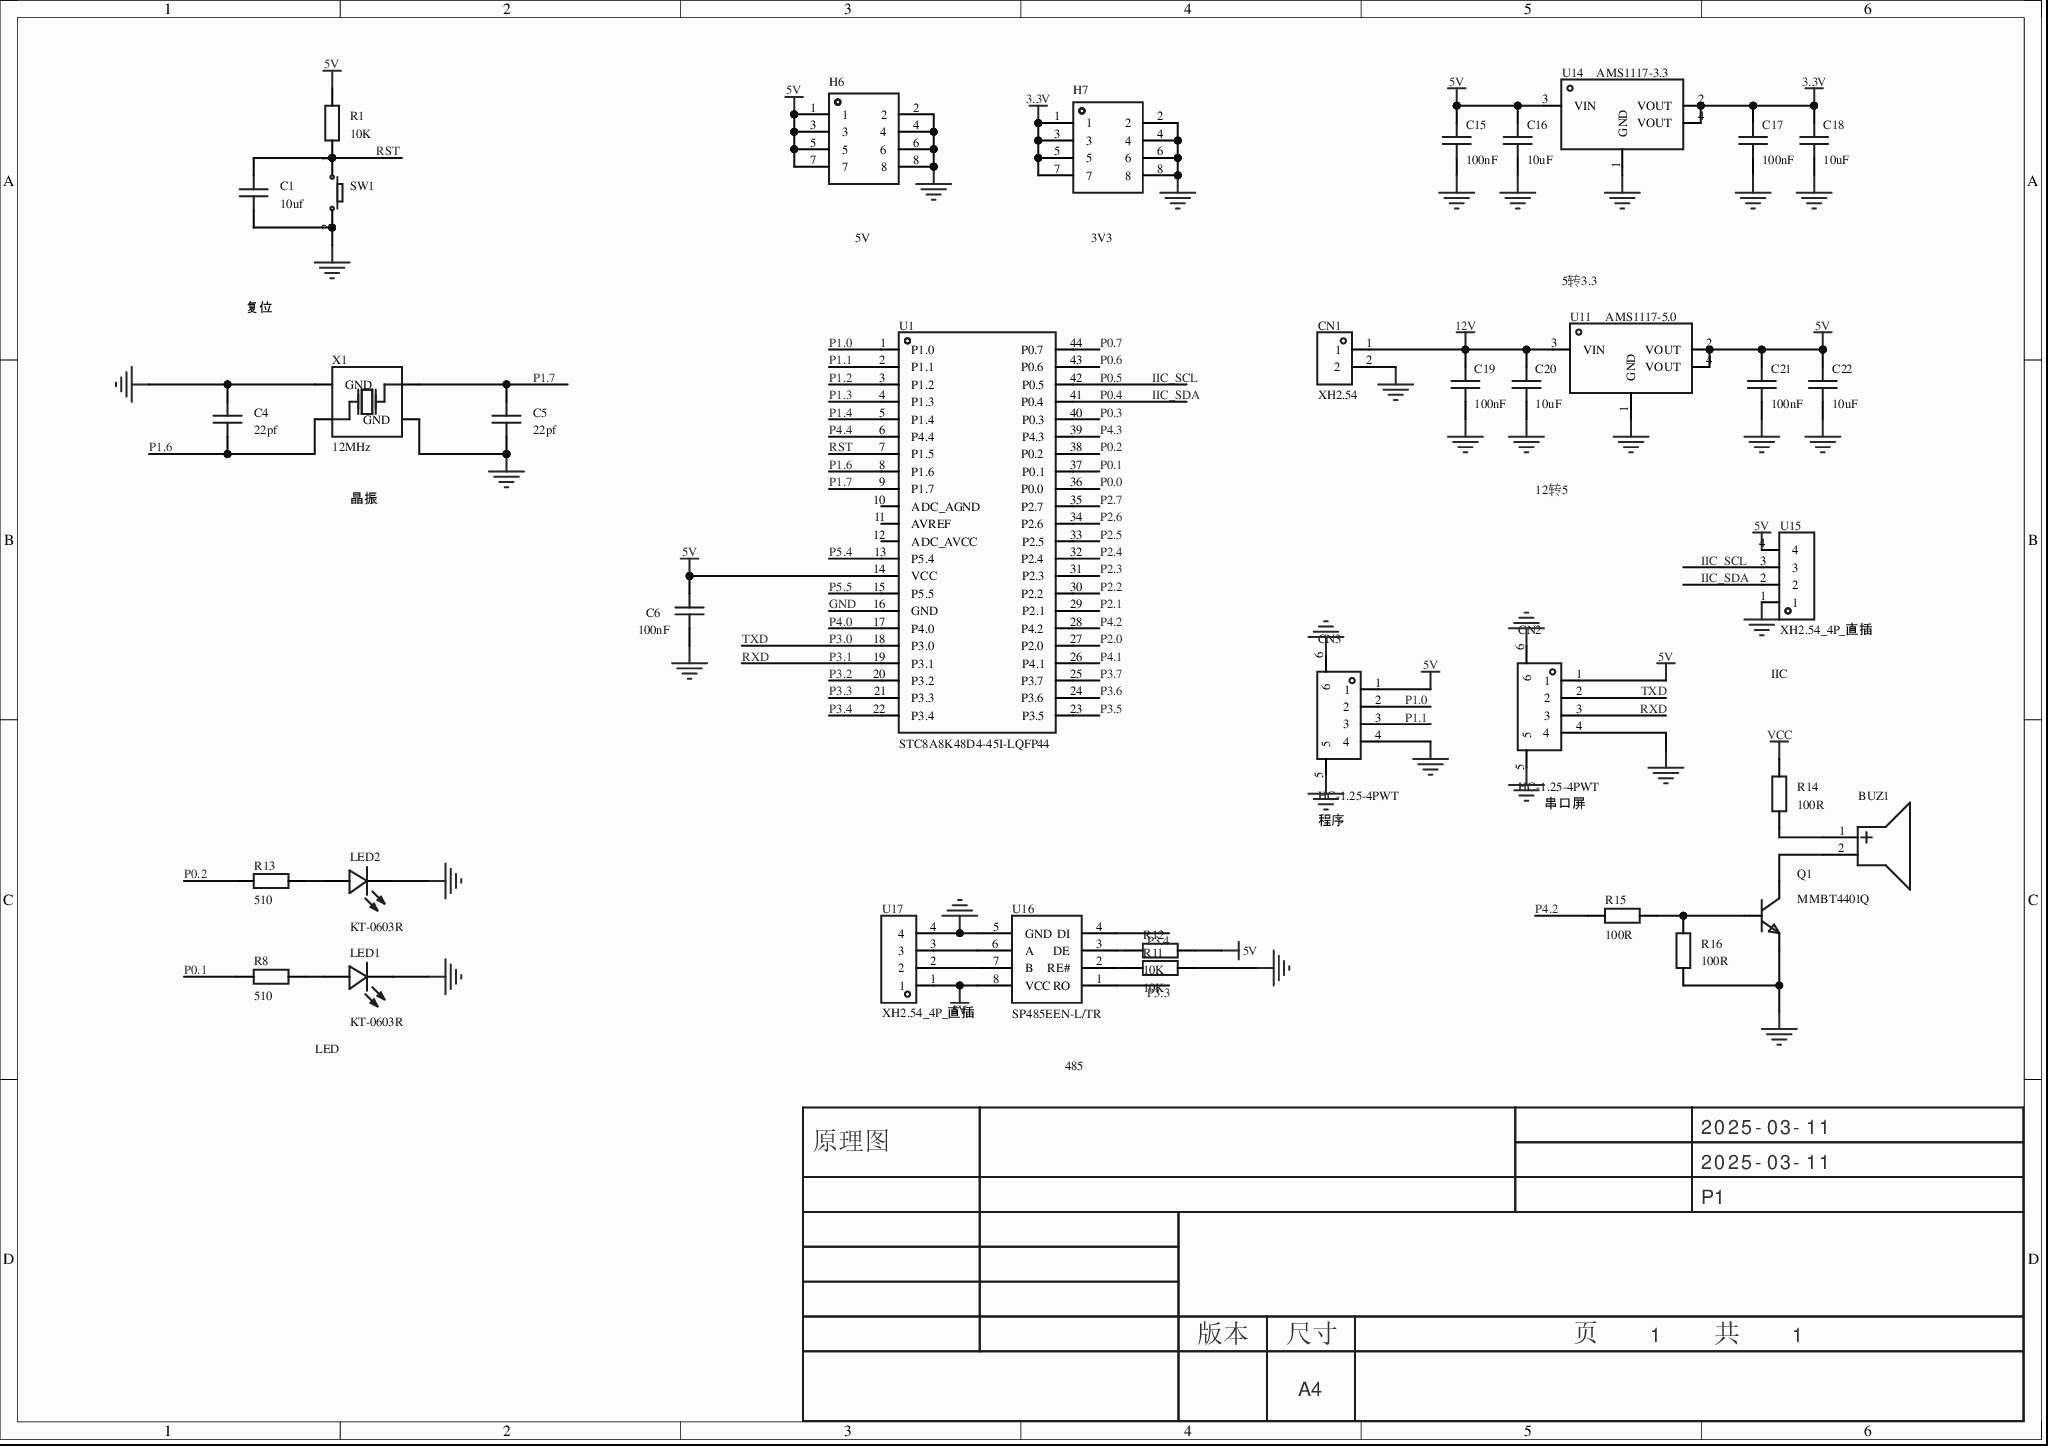
[diagram p0: MISC49860-3.schdoc]
# Altium project MISC49860-2.PrjPcb
1 sheet, 37 parts. Net scope: global (net labels, ports and power ports of the same name join across sheets).
Board file: MISC49860.pcbdoc

## Sheet MISC49860-3.schdoc
size 297 x 209 mm; Version: V1.0; @Project Name: MISC49860; @Page Count: 1; @Update Date: 2025-03-11; @Create Date: 2025-03-11; @Schematic Name: MISC49860; @Page No: 1; @Create Time: 19:24:41; @Update Time: 19:59:04; @Board Name: MISC49860

### Parts
BUZ1  5VDC蜂鸣器,Φ12,脚距7.6  [BUZ-TH_BD12.0-P7.60-D0.6-FD]  (value not drawn)
C1  10uf  [C0805]
C4  22pf  [C0805]
C5  22pf  [C0805]
C6  100nF  [C0805]
C15  100nF  [C0603]
C16  10uF  [C0603]
C17  100nF  [C0603]
C18  10uF  [C0603]
C19  100nF  [C0603]
C20  10uF  [C0603]
C21  100nF  [C0603]
C22  10uF  [C0603]
CN1  XH2.54  [CONN-TH_XH2.54-2P]
CN2  HC-1.25-4PWT  [CONN-SMD_4P-P1.25-HC-1.25-4PWT]
CN3  HC-1.25-4PWT  [CONN-SMD_4P-P1.25-HC-1.25-4PWT]
H6  (no value)  [HDR-TH_8P-P2.54-V-M-R2-C4-S2.54]
H7  (no value)  [HDR-TH_8P-P2.54-V-M-R2-C4-S2.54]
LED1  KT-0603R  [LED0603-RD]
LED2  KT-0603R  [LED0603-RD]
Q1  MMBT4401Q  [SOT-23-3_L2.9-W1.3-P1.90-LS2.4-BR]
R1  10K  [R0805]
R8  510  [R0603]
R11  10K  [R0805]
R12  10K  [R0805]
R13  510  [R0603]
R14  100R  [R0805]
R15  100R  [R0805]
R16  100R  [R0805]
SW1  (no value)  [Key_SMD_3x4x2]
U1  STC8A8K48D4-45I-LQFP44  [LQFP-44_L10.0-W10.0-P0.80-LS12.0-BL]
U11  AMS1117-5.0  [SOT-223_L6.5-W3.5-P2.30-LS7.0-BR]
U14  AMS1117-3.3  [SOT-223-3_L6.5-W3.4-P2.30-LS7.0-BR]
U15  XH2.54_4P_直插  [CONN-TH_4P-P2.50-XH2.54-4P]
U16  SP485EEN-L/TR  [SOIC-8_L5.0-W4.0-P1.27-LS6.0-BL]
U17  XH2.54_4P_直插  [CONN-TH_4P-P2.50-XH2.54-4P]
X1  12MHz  [OSC-SMD_4P-L3.2-W2.5-BL]

### Nets
3.3V: C17.2 C18.2 H7.1 H7.3 H7.5 H7.7 U14.2(VOUT) U14.4(VOUT)
5V: C6.2 C15.2 C16.2 C21.2 C22.2 CN2.1 CN3.1 H6.1 H6.3 H6.5 H6.7 R1.1 R12.2 U1.14(VCC) U11.2(VOUT) U11.4(VOUT) U14.3(VIN) U15.4 U16.8(VCC) U17.1
12V: C19.2 C20.2 CN1.1 U11.3(VIN)
GND: C1.2 C4.2 C5.1 C6.1 C15.1 C16.1 C17.1 C18.1 C19.1 C20.1 C21.1 C22.1 CN1.2 CN2.4 CN2.5 CN2.6 CN3.4 CN3.5 CN3.6 H6.2 H6.4 H6.6 H6.8 H7.2 H7.4 H7.6 H7.8 LED1.1(K) LED2.1(K) Q1.2(E) R11.2 R16.2 SW1.2 U1.16(GND) U11.1(GND) U14.1(GND) U15.1 U16.5(GND) U17.4 X1.2(GND) X1.4(GND)
VCC: R14.1
IIC_SCL: U1.42(P0.5) U15.3  [also labelled P0.5]
IIC_SDA: U1.41(P0.4) U15.2  [also labelled P0.4]
P0.0: U1.36(P0.0)
P0.1: R8.1 U1.37(P0.1)
P0.2: R13.1 U1.38(P0.2)
P0.3: U1.40(P0.3)
P0.6: U1.43(P0.6)
P0.7: U1.44(P0.7)
P1.0: CN3.2 U1.1(P1.0)
P1.1: CN3.3 U1.2(P1.1)
P1.2: U1.3(P1.2)
P1.3: U1.4(P1.3)
P1.4: U1.5(P1.4)
P1.6: C4.1 U1.8(P1.6) X1.1(OSC1)
P1.7: C5.2 U1.9(P1.7) X1.3(OSC2)
P2.0: U1.27(P2.0)
P2.1: U1.29(P2.1)
P2.2: U1.30(P2.2)
P2.3: U1.31(P2.3)
P2.4: U1.32(P2.4)
P2.5: U1.33(P2.5)
P2.6: U1.34(P2.6)
P2.7: U1.35(P2.7)
P3.0: CN2.2 U1.18(P3.0)  [also labelled TXD]
P3.1: CN2.3 U1.19(P3.1)  [also labelled RXD]
P3.2: U1.20(P3.2)
P3.3: U1.21(P3.3) U16.1(RO)
P3.4: U1.22(P3.4) U16.4(DI)
P3.5: U1.23(P3.5)
P3.6: U1.24(P3.6)
P3.7: U1.25(P3.7)
P4.0: U1.17(P4.0)
P4.1: U1.26(P4.1)
P4.2: R15.1 U1.28(P4.2)
P4.3: U1.39(P4.3)
P4.4: U1.6(P4.4)
P5.4: U1.13(P5.4)
P5.5: U1.15(P5.5)
RST: C1.1 R1.2 SW1.1 U1.7(P1.5)
NetBUZ1_1: BUZ1.1(+) R14.2
NetBUZ1_2: BUZ1.2(-) Q1.3(C)
NetLED1_2: LED1.2(A) R8.2
NetLED2_2: LED2.2(A) R13.2
NetQ1_1: Q1.1(B) R15.2 R16.1
NetR11_1: R11.1 U16.2(RE#)
NetR12_1: R12.1 U16.3(DE)
NetU16_6: U16.6(A) U17.3
NetU16_7: U16.7(B) U17.2

Not connected (* = marked no-connect by the designer): U1 10(ADC_AGND) 11(AVREF) 12(ADC_AVCC)

### Notes on the sheet
- (near H6) 5V
- (near H7) 3V3
- 复位
- 5转3.3
- 晶振
- 12转5
- IIC
- (near CN3) 程序
- (near CN2) 串口屏
- LED
- 485
- 2025-03-11
- 原理图
- P1
- 版本
- 尺寸
- A4
- 页    1    共    1

### Library data of the parts
BUZ1 = 5VDC蜂鸣器,Φ12,脚距7.6: AddInBom: yes; ModelId: 16ab50e14c5b4f2c986c135bdba60e37; ModelName: BUZ-TH_D12.0-H9.5-P7.60; ModelTransform: 472.44,472.176,0,90,0,0,-0.787,0,-177.165; Symbol: 5VDC蜂鸣器,Φ12,脚距7.6; Device: 5VDC蜂鸣器,Φ12,脚距7.6; LCSC Part Name: 5VDC蜂鸣器,Φ12,脚距7.6; SupplierPart: C9900018824; ManufacturerPart: 5VDC蜂鸣器,Φ12,脚距7.6; Supplier Footprint: BUZ-TH; JLCPCB Part Class: 扩展库; Supplier: LCSC; ConvertToPcb: yes; FootprintName: BUZ-TH_BD12.0-P7.60-D0.6-FD
C1 C4-C6 = CAP_0805: ConvertToPcb: yes; SymbolName: CapAcitance; ModelId: 1ba041120af144c991958decab20d241; ModelName: C0805_L2.0-W1.3-H1.3; ModelTransform: 78.74,51.181,0,0,0,0,0,0.0005,0; Device: CAP_0805; AddInBom: yes; Supplier Footprint: 0805; FootprintName: C0805
  C1: Value: 10uf
  C4 C5: Value: 22pf
  C6: Value: 100nF
C15-C22 = CAP_0603: ConvertToPcb: yes; SymbolName: CapAcitance; ModelId: ac125912035d415993ca9572d50418b1; ModelName: C0603_L1.6-W0.8-H0.8; ModelTransform: 62.992,31.496,0,0,0,0,0,0,0; Device: CAP_0603; AddInBom: yes; Supplier Footprint: 0603; FootprintName: C0603
  C15 C17 C19 C21: Value: 100nF
  C16 C18 C20 C22: Value: 10uF
CN1 = XH2.54-2PIN-直针: AddInBom: yes; ModelId: dc9654a6caad4c20aab3bc231ea458cf; ModelTransform: 296.889,230.315,0,0,0,0,0,26.653,-137.795; Symbol: XH2.54-2PIN-直针; Manufacturer Part: XH2.54; Device: XH2.54-2PIN-直针; LCSC Part Name: XH2.54-2PIN-直针; SupplierPart: C9900011425; Supplier Footprint: XH2.54-2PIN; JLCPCB Part Class: 扩展库; Supplier: LCSC; ConvertToPcb: yes; FootprintName: CONN-TH_XH2.54-2P; ModelName: CONN-TH_XH2.54-2P
CN2 CN3 = HC-1.25-4PWT: 插针结构:1x4P;间距:1.25mm;安装方式:卧贴;参考系列:PicoBlade(MX 1.25);总PIN数:4P;排数:1;每排PIN数:4;行距:-;额定电流:1A;触头材质:黄铜;触头镀层:锡;工作温度范围:-40℃~+105℃;; Manufacturer: HCTL(华灿天禄); AddInBom: yes; ModelId: a5d89d01fe1c41f780224f4e5aebbf3c; ModelTransform: 393.7,206.693,0,0,0,0,-0.001,-39.372,0; Pins Structure: 1x4P; Pitch: 1.25mm; Number of PINs Per Row: 4; Current Rating (Max): 1A; Rated Voltage (Max): 125V; Plastic Material: LCP; Flame Retardant Rating: UL94V-0; Supplementary Features: 辅助焊脚; Z-Height of the Board: 3.57mm; X-Length of Bottom Edge on Board (Spacing Line): 10.05mm; Y-Width of Bottom Edge on Board: 5.25mm; Symbol: HC-1.25-4PWT; Device: HC-1.25-4PWT; LCSC Part Name: 1x4P 间距:1.25mm 卧贴 系列:PicoBlade(MX 1.25); SupplierPart: C2845381; ManufacturerPart: HC-1.25-4PWT; Supplier Footprint: SMD,P=1.25mm,卧贴; JLCPCB Part Class: 扩展库; Datasheet: https://atta.szlcsc.com/upload/public/pdf/source/20240930/9508A8292CCC87B0C29E3A028D56E30A.pdf; Supplier: LCSC; ConvertToPcb: yes; FootprintName: CONN-SMD_4P-P1.25-HC-1.25-4PWT; ModelName: CONN-SMD_4P-P1.25-HC-1.25-4PWT; Mounting Style: 卧贴; Reference Series: PicoBlade(MX 1.25); Number of Pins: 4P; Number of Rows: 1; Row Spacing: -; Contact Material: 黄铜; Contact Plating: 锡; Operating Temperature Range: -40℃~+105℃; Colour: -
H6 H7 = HDR-M_2.54_2x4: Symbol: HDR-M-2.54_2x4; ConvertToPcb: yes; ModelId: 9655140a9899454ea9d6a6732d55fb0e; ModelName: HDR-TH_8P-P2.54-M-LI-2X4P; ModelTransform: 399.999,200,0,0,0,0,0,0,-118.11; Device: HDR-M_2.54_2x4; AddInBom: yes; SupplierPart: C124386; Supplier Footprint: 插件,P=2.54mm; FootprintName: HDR-TH_8P-P2.54-V-M-R2-C4-S2.54
LED1 LED2 = KT-0603R: 发光颜色:红色;功率:-;正向电流:-;主波长:-;二极管配置:-;透镜颜色:-;色温:-;发光角度:-;载带方式:-;工作温度:-40℃~+85℃;; Manufacturer: KENTO; AddInBom: yes; ModelId: 1f0d29a91be547639d425604e9b96ebb; ModelTransform: 63.7794,32.283,0,0,0,0,0,0,0; Emitted Color: 红色; Symbol: KT-0603R; Device: KT-0603R; LCSC Part Name: 0603 红灯 高亮; SupplierPart: C2286; ManufacturerPart: KT-0603R; Supplier Footprint: 0603; JLCPCB Part Class: 基础库; Datasheet: https://atta.szlcsc.com/upload/public/pdf/source/20160616/1466072038404.pdf; Supplier: LCSC; ConvertToPcb: yes; FootprintName: LED0603-RD; ModelName: LED0603-RD; Power Dissipation: -; Forward Current: -; Dominant Wavelength: -; Peak Wavelength: -; Diode Configuration: -; Lens Color: -; Color Temperature: -; Viewing Angle: -; Mounting Sytle: -; Operating Temperature: -40℃~+85℃
Q1 = MMBT4401Q: 晶体管类型:NPN;集电极电流(Ic):600mA;集射极击穿电压(Vceo):40V;耗散功率(Pd):300mW;直流电流增益(hFE):100@150mA,1V;; Manufacturer: YANGJIE(扬杰); AddInBom: yes; ModelId: c62791f0466c4ae2a892c056b845b0ca; ModelName: SOT-23-3P_L2.9-W1.3-H1.0-LS2.4-P0.95; ModelTransform: 98.425,114.173,0,180,0,0,0.0005,-0.0005,0; type: NPN; Current - Collector(Ic): 600mA; Collector - Emitter Voltage VCEO: 40V; Pd - Power Dissipation: 300mW; Transition frequency(fT): 250MHz; Current - Collector Cutoff: 100nA; Vce Saturation(VCE(sat)): 400mV@150mA,15mA; Symbol: MMBT4401Q; Device: MMBT4401Q; LCSC Part Name: MMBT4401Q; SupplierPart: C699219; ManufacturerPart: MMBT4401Q; Supplier Footprint: SOT-23(TO-236); JLCPCB Part Class: 扩展库; Datasheet: https://atta.szlcsc.com/upload/public/pdf/source/20200709/C699219_5916070C8AE9E936AEED1A6139F8D2E4.pdf; Supplier: LCSC; ConvertToPcb: yes; FootprintName: SOT-23-3_L2.9-W1.3-P1.90-LS2.4-BR; DC Current Gain: 100@150mA,1V; Operating Temperature: -55℃~+150℃
R1 R11 R12 R14-R16 = Res_0805: Symbol: 电阻; ConvertToPcb: yes; ModelId: 37a81e68749a4138bd2dfa6897b24b85; ModelName: R0805_L2.0-W1.3-H0.6; ModelTransform: 78.74,51.181,0,0,0,0,0,-0.0005,0; Device: Res_0805; AddInBom: yes; Supplier Footprint: 0805; FootprintName: R0805
  R1 R11 R12: Value: 10K
  R14-R16: Value: 100R
R8 R13 = Res_0603: ConvertToPcb: yes; SymbolName: 电阻; ModelId: fc143cca1e79419f9cd78b61e9279f08; ModelTransform: 31.8897,63.7794,0,90,0,0,0,0,0; Value: 510; Device: Res_0603; AddInBom: yes; Supplier Footprint: 0603; FootprintName: R0603; ModelName: R0603
SW1 = Key_SMD_3x4x2: ConvertToPcb: yes; SymbolName: 轻触按键x2; ModelId: 63599cce708d48afbce1b0db003544770819f05c4eef4c71ace90d822a990e87; ModelName: SW-SMD_L4.0-W2.9-H2-LS5.0; ModelTransform: 196.85,114.17,79.13,0,0,0,0,0,0; Device: Key_SMD_3x4x2; AddInBom: yes; Supplier Footprint: SMD; FootprintName: Key_SMD_3x4x2
U1 = STC8A8K48D4-45I-LQFP44: Manufacturer: STC(宏晶); AddInBom: yes; ModelId: cfc67ede9fd147078f17820e55193bca; ModelName: LQFP-44_L10.0-W10.0-H1.4-LS12.0-P0.80; ModelTransform: 472.441,472.441,0,0,0,0,0,0,0; Symbol: STC8A8K48D4-45I-LQFP44; Device: STC8A8K48D4-45I-LQFP44; LCSC Part Name: STC8A8K48D4-45I-LQFP44; SupplierPart: C3013132; ManufacturerPart: STC8A8K48D4-45I-LQFP44; Supplier Footprint: LQFP-44(10x10); JLCPCB Part Class: 扩展库; Datasheet: https://atta.szlcsc.com/upload/public/pdf/source/20220509/6F36F3B8C41E8D6E23754E39225582EF.pdf; Supplier: LCSC; ConvertToPcb: yes; FootprintName: LQFP-44_L10.0-W10.0-P0.80-LS12.0-BL
U11 = AMS1117-5.0_C6187: 输出类型:固定;工作电压:12V;输出电压:5V;输出电流:1A;电源纹波抑制比(PSRR):-;输出极性:正极;; Manufacturer: AMS; AddInBom: yes; Output Type: 固定; Voltage - Supply: 12V; Output Voltage: 5V; Output Current: 1A; Voltage Dropout: 1.3V@(1A); Output Configuration: 正极; Number of Outputs: 1; ModelId: 925194bf9823436183a3e0b978a8d076; ModelName: SOT-223-4P_L6.5-W3.5-H1.6-LS7.0-P2.30; ModelTransform: 279.89794,255.905,0,180,0,0,0.0005,0.0005,0; Symbol: AMS1117-5.0; Device: AMS1117-5.0_C6187; LCSC Part Name: 输入12V 输出5V 1A; SupplierPart: C6187; ManufacturerPart: AMS1117-5.0; Supplier Footprint: SOT-223; JLCPCB Part Class: 基础库; Datasheet: https://atta.szlcsc.com/upload/public/pdf/source/20230918/E4B716057EE82179D88E8A0894830D59.pdf; Supplier: LCSC; ConvertToPcb: yes; Power Supply Rejection Ratio (PSRR): -; standby current: -; Noise: -; Features: 过流保护(OCP); Operating Temperature: -; FootprintName: SOT-223_L6.5-W3.5-P2.30-LS7.0-BR
U14 = AMS1117-3.3_C6186: 输出类型:固定;工作电压:-;输出电压:3.3V;输出电流:1A;电源纹波抑制比(PSRR):72dB@(120Hz);输出极性:正极;; Manufacturer: AMS; AddInBom: yes; Output Type: 固定; Output Voltage: 3.3V; Output Current: 1A; Voltage Dropout: 1.3V@(800mA); Output Configuration: 正极; Number of Outputs: 1; ModelId: 925194bf9823436183a3e0b978a8d076; ModelName: SOT-223-4P_L6.5-W3.5-H1.6-LS7.0-P2.30; ModelTransform: 279.89794,255.905,0,180,0,0,-3.9385,-0.0005,0; Symbol: AMS1117-3.3; Device: AMS1117-3.3_C6186; LCSC Part Name: 输出3.3V 1A; SupplierPart: C6186; ManufacturerPart: AMS1117-3.3; Supplier Footprint: SOT-223; Datasheet: https://atta.szlcsc.com/upload/public/pdf/source/20180727/C6186_7A095716F0823C02F1997A905E26C086.pdf; Supplier: LCSC; ConvertToPcb: yes; Voltage - Supply: -; Power Supply Rejection Ratio (PSRR): 72dB@(120Hz); standby current: -; Noise: -; Features: 过流保护(OCP)；热关断(TSD); Operating Temperature: -; FootprintName: SOT-223-3_L6.5-W3.4-P2.30-LS7.0-BR
U15 U17 = XH2.54_4P_直插: AddInBom: yes; ModelId: c69236e4c0a047c6aeeeefc1552045f5; ModelTransform: 492.125,228.346,0,180,0,0,0,-19.685,-137.795; Symbol: XH2.54_4P_直插; Device: XH2.54_4P_直插; LCSC Part Name: XH2.54_4P_直插; SupplierPart: C9900008616; ManufacturerPart: XH2.54_4P_直插; Supplier Footprint: XH2.54_4P; JLCPCB Part Class: 扩展库; Supplier: LCSC; ConvertToPcb: yes; FootprintName: CONN-TH_4P-P2.50-XH2.54-4P; ModelName: CONN-TH_4P-P2.50-XH2.54-4P
U16 = SP485EEN-L/TR: 类型:收发器;数据速率:10Mbps;; Manufacturer: MaxLinear(迈凌); AddInBom: yes; ModelId: e81d2f7d937b4a6ab1dca543ff5d56a4; ModelName: SOIC-8_L4.9-W3.9-H1.7-LS6.0-P1.27; ModelTransform: 189.751,236.22,0,0,0,0,-0.0005,0.0005,0; Types: 收发器; Number of Driver: 1; Supply Voltage: 4.75V~5.25V; Data Rate: 10Mbps; Symbol: SP485EEN-L/TR; Device: SP485EEN-L/TR; LCSC Part Name: 增强型低功耗半双工 RS-485 收发器; SupplierPart: C6855; ManufacturerPart: SP485EEN-L/TR; Supplier Footprint: SOIC-8; Datasheet: https://atta.szlcsc.com/upload/public/pdf/source/20210125/C916163_66C97B5ACCC910994E8B10780F9BD300.pdf; Supplier: LCSC; ConvertToPcb: yes; FootprintName: SOIC-8_L5.0-W4.0-P1.27-LS6.0-BL; Number of receiver: 1; Operating Temperature: -40℃~+85℃
X1 = 7M12000039: 晶振类型:贴片晶振;频率:12MHz;常温频差:±20ppm;外接负载电容:18pF;频率稳定度(全温):±20ppm;; Manufacturer: TXC(晶技); Symbol: 7M1209LCSC-DDJ4S; AddInBom: yes; ModelId: ae22b8d143894765bc8100c37cb6356f; ModelName: OSC-SMD_4P-L3.2-W2.5-H1.0; ModelTransform: 125.984,98.425,0,0,0,0,0,0,0; Crystal Type: 贴片晶振; Normal temperature Frequency Tolerance: ±20ppm; External load capacitor: 18pF; Equivalent Series Resistance (ESR): 100Ω; Device: 7M12000039; LCSC Part Name: 12MHz ±20ppm 18pF; SupplierPart: C90900; ManufacturerPart: 7M12000039; Supplier Footprint: SMD3225-4P; JLCPCB Part Class: 扩展库; Datasheet: https://atta.szlcsc.com/upload/public/pdf/source/20170408/1491621572265.pdf; Supplier: LCSC; ConvertToPcb: yes; FootprintName: OSC-SMD_4P-L3.2-W2.5-BL; Value: 12MHz; Frequency Stability(Full temperature range): ±20ppm; Operating Temperature: -10℃~+70℃